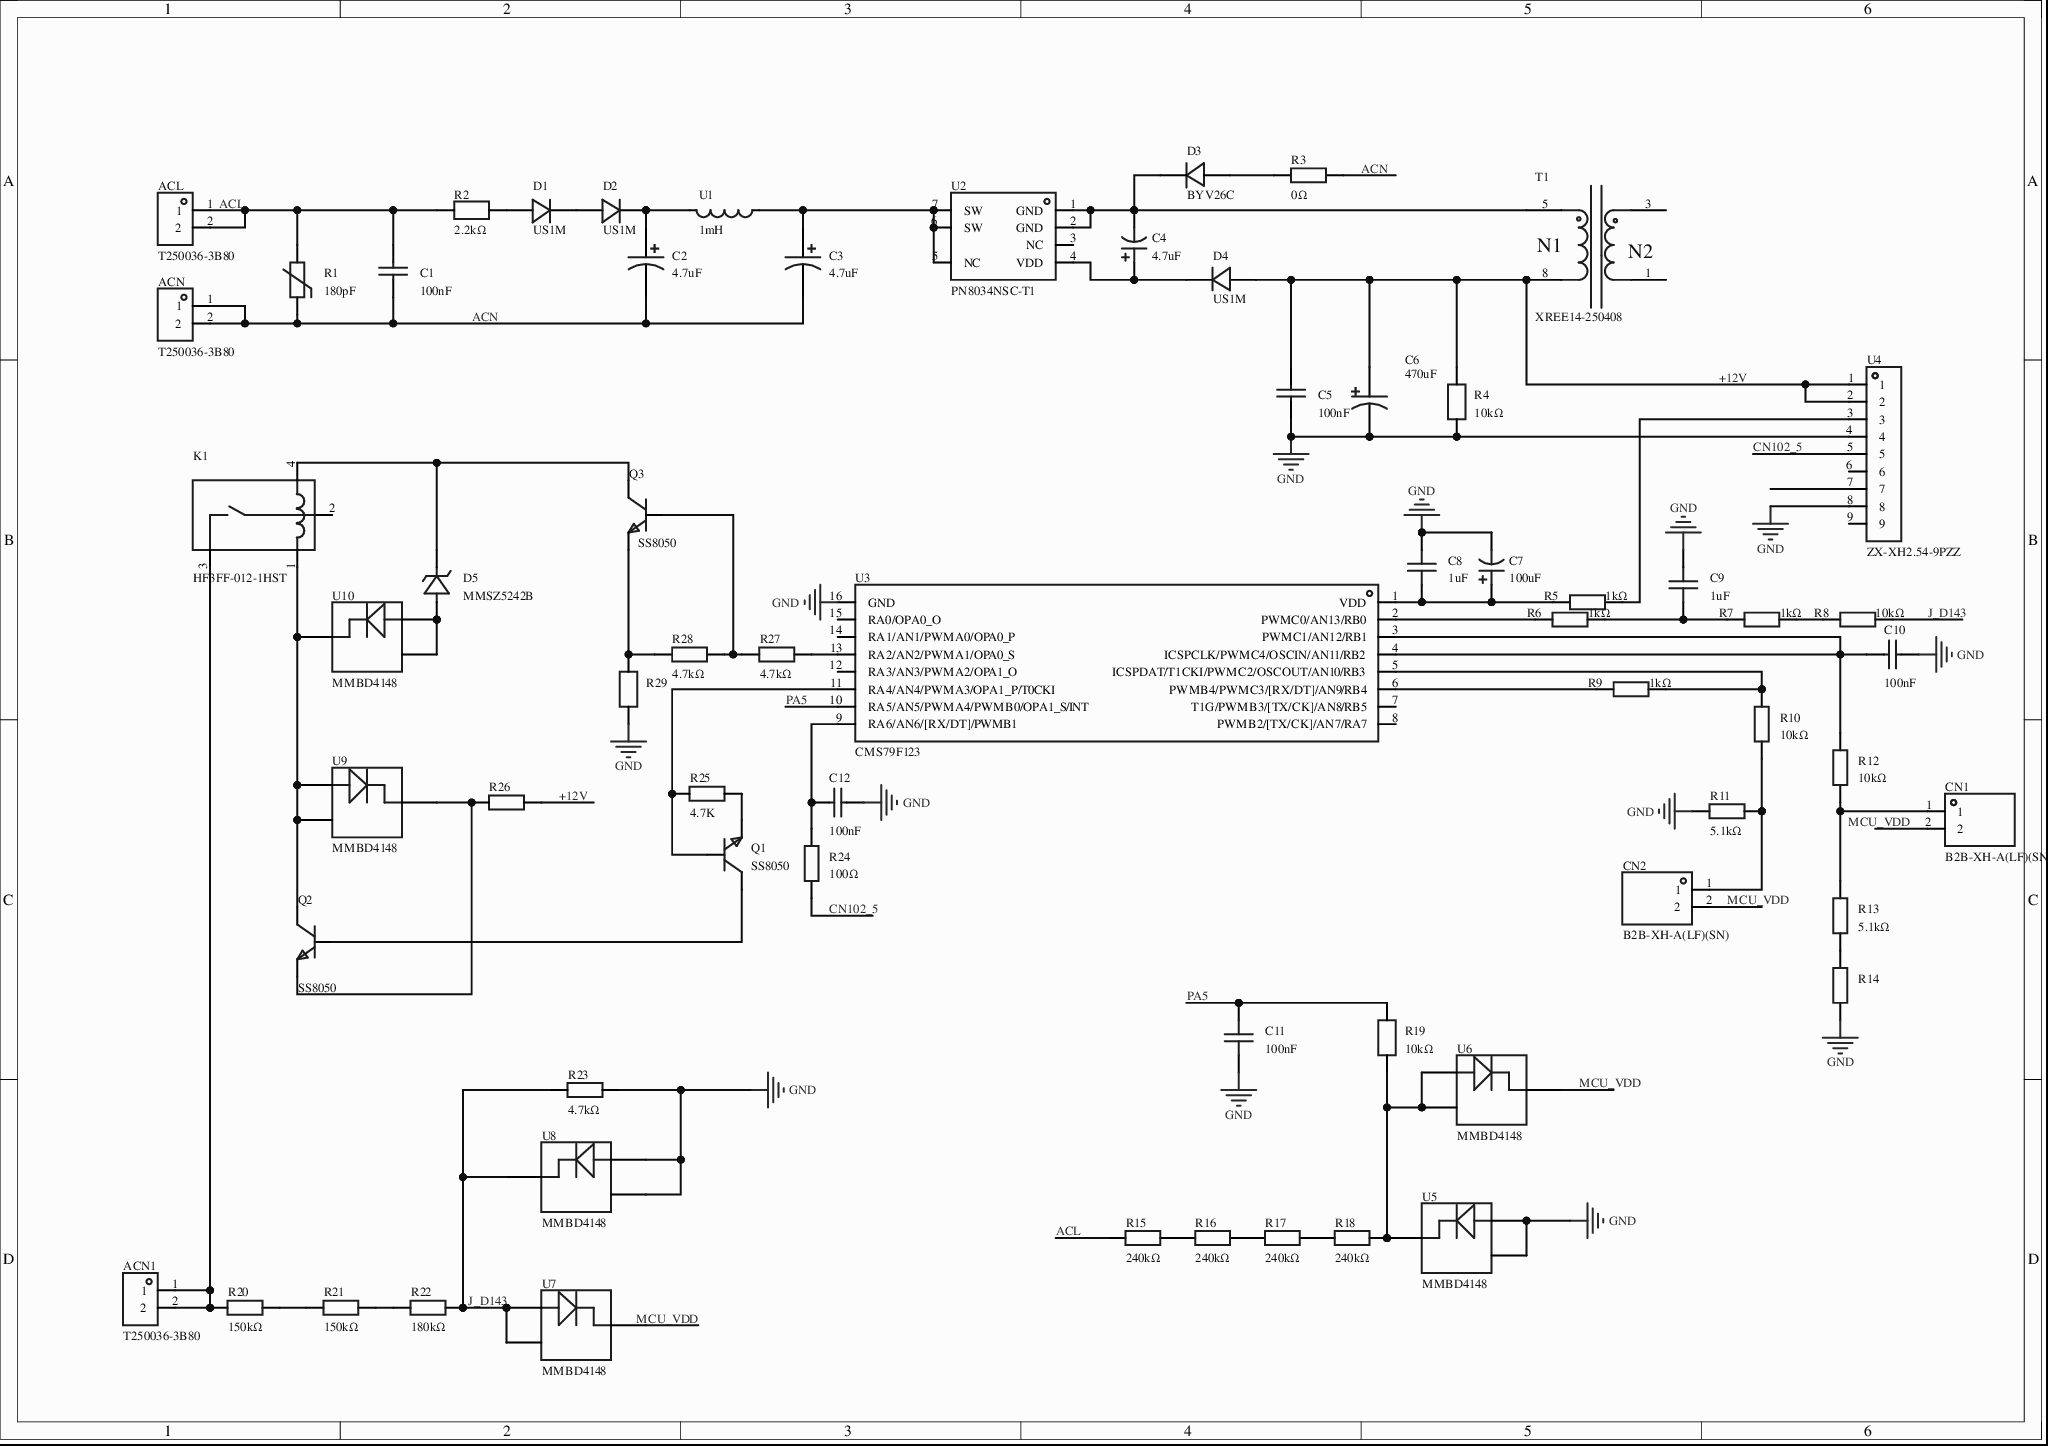
[diagram p0: MISC51809-3.schdoc]
# Altium project MISC51809-2.PrjPcb
1 sheet, 66 parts. Net scope: global (net labels, ports and power ports of the same name join across sheets).
Board file: MISC51809.pcbdoc

## Sheet MISC51809-3.schdoc
size 297 x 209 mm; Version: V1.0; @Project Name: MISC51809; @Update Date: 2026-04-03; @Create Date: 2026-04-03; @Board Name: MISC51809; @Create Time: 12:09:30; @Page Count: 1; @Page No: 1; @Schematic Name: MISC51809; @Update Time: 12:09:30; Size: A4

### Parts
ACL  T250036-3B80  [CONN-TH_XFCN-T250036-3B80]
ACN  T250036-3B80  [CONN-TH_XFCN-T250036-3B80]
ACN1  T250036-3B80  [CONN-TH_XFCN-T250036-3B80]
C1  100nF  [CAP-TH_L18.0-W6.0-P15.00-D1.2]
C2  4.7uF  [CAP-TH_BD10.0-P5.00-D1.0-FD]
C3  4.7uF  [CAP-TH_BD10.0-P5.00-D1.0-FD]
C4  4.7uF  [CAP-TH_BD6.3-P2.50-D0.5-FD]
C5  100nF  [C0603]
C6  470uF  [CAP-TH_BD10.0-P5.00-D1.0-FD]
C7  100uF  [CAP-TH_BD6.3-P2.50-D0.5-FD]
C8  1uF  [C0603]
C9  1uF  [C0603]
C10  100nF  [C0603]
C11  100nF  [C0603]
C12  100nF  [C0603]
CN1  B2B-XH-A(LF)(SN)  [CONN-TH_B2B-XH-A-LF-SN]
CN2  B2B-XH-A(LF)(SN)  [CONN-TH_B2B-XH-A-LF-SN]
D1  US1M  [SMA_L4.4-W2.8-LS5.4-RD]
D2  US1M  [SMA_L4.4-W2.8-LS5.4-RD]
D3  BYV26C  [SMA_L4.4-W2.6-LS5.1-FD]
D4  US1M  [SMA_L4.4-W2.8-LS5.4-RD]
D5  MMSZ5242B  [SOD-123_L2.7-W1.6-LS3.7-RD]
K1  HF3FF-012-1HST  [RELAY-TH_HF3FF-012-1HST]
Q1  SS8050  [SOT-23-3_L2.9-W1.3-P1.90-LS2.4-BR]
Q2  SS8050  [SOT-23-3_L2.9-W1.3-P1.90-LS2.4-BR]
Q3  SS8050  [SOT-23-3_L2.9-W1.3-P1.90-LS2.4-BR]
R1  180pF  [RES-TH_L11.0-W5.5-P7.50-D0.8-S4.70]
R2  2.2kΩ  [RES-TH_BD4.5-L11.5-P15.50-D0.8]
R3  0Ω  [R0805]
R4  10kΩ  [R0603]
R5  1kΩ  [R0603]
R6  1kΩ  [R0603]
R7  1kΩ  [R0603]
R8  10kΩ  [R0603]
R9  1kΩ  [R0603]
R10  10kΩ  [R0603]
R11  5.1kΩ  [R0603]
R12  10kΩ  [R0603]
R13  5.1kΩ  [R0603]
R14  1kΩ  [R0603]  (value not drawn)
R15  240kΩ  [R0805]
R16  240kΩ  [R0805]
R17  240kΩ  [R0805]
R18  240kΩ  [R0805]
R19  10kΩ  [R0603]
R20  150kΩ  [R0805]
R21  150kΩ  [R0805]
R22  180kΩ  [R0805]
R23  4.7kΩ  [RES-TH_BD3.3-L9.0-P13.00-D0.6]
R24  100Ω  [R0603]
R25  4.7K  [R0603]
R26  4.7K  [R0603]  (value not drawn)
R27  4.7kΩ  [R0603]
R28  4.7kΩ  [R0603]
R29  10kΩ  [R0603]  (value not drawn)
T1  XREE14-250408  [XFMR-TH_XREE14-250408]
U1  1mH  [IND-TH_BD3.0-L8.0-P12.00-D0.6]
U2  PN8034NSC-T1  [DIP-8_7P-L9.3-W6.4-P2.54-LS7.6-BL-PE6]
U3  CMS79F123  [SOPN-16_L9.9-W3.9-P1.27-LS6.0-BL]
U4  ZX-XH2.54-9PZZ  [CONN-TH_9P-P2.50_ZX-XH2.54-9PZZ]
U5  MMBD4148  [SOT-23-3_L2.9-W1.3-P1.90-LS2.4-BR]
U6  MMBD4148  [SOT-23-3_L2.9-W1.3-P1.90-LS2.4-BR]
U7  MMBD4148  [SOT-23-3_L2.9-W1.3-P1.90-LS2.4-BR]
U8  MMBD4148  [SOT-23-3_L2.9-W1.3-P1.90-LS2.4-BR]
U9  MMBD4148  [SOT-23-3_L2.9-W1.3-P1.90-LS2.4-BR]
U10  MMBD4148  [SOT-23-3_L2.9-W1.3-P1.90-LS2.4-BR]

### Nets
GND: C5.1 C6.2 C7.2 C8.2 C9.2 C10.1 C11.1 C12.2 R4.1 R11.2 R14.1 R23.2 R29.1 U3.16(GND) U4.4 U4.8 U5.1 U5.2 U8.1 U8.2
+12V: C5.2 C6.1 D4.2(A) R4.2 R26.2 T1.8 U4.1 U4.2
ACL: ACL.1 ACL.2 C1.2 R1.2 R2.1 R15.1
ACN: ACN.1 ACN.2 C1.1 C2.2 C3.2 R1.1 R3.2
CN102_5: R24.1 U4.5
J_D143: R8.2 R22.2 R23.1 U7.1 U7.2 U8.3
MCU_VDD: CN1.2 CN2.2 U6.3 U7.3
PA5: C11.2 R19.2 U3.10(RA5/AN5/PWMA4/PWMB0/OPA1_S/INT)
NetACN1_1: ACN1.1 ACN1.2 K1.3 R20.1
NetC2_1: C2.1 D2.1(C) U1.1
NetC3_1: C3.1 U1.2 U2.5(NC) U2.6(SW) U2.7(SW)
NetC4_1: C4.1 D4.1(C) U2.4(VDD)
NetC4_2: C4.2 D3.2 T1.5 U2.1(GND) U2.2(GND)
NetC7_1: C7.1 C8.1 R5.1 U3.1(VDD)
NetC9_1: C9.1 R6.2 R7.1
NetC10_2: C10.2 R12.2 U3.3(PWMC1/AN12/RB1) U3.4(ICSPCLK/PWMC4/OSCIN/AN11/RB2)
NetC12_1: C12.1 R24.2 U3.9(RA6/AN6/[RX/DT]/PWMB1)
NetCN1_1: CN1.1 R12.1 R13.1
NetCN2_1: CN2.1 R10.1 R11.1
NetD1_1: D1.1(C) D2.2(A)
NetD1_2: D1.2(A) R2.2
NetD3_1: D3.1 R3.1
NetD5_1: D5.1(K) K1.4 Q3.3(C)
NetD5_2: D5.2(A) U10.1 U10.2
NetK1_1: K1.1 Q2.3(C) U9.1 U9.2 U10.3
NetQ1_1: Q1.1(B) R25.1 U3.11(RA4/AN4/PWMA3/OPA1_P/T0CKI)
NetQ1_2: Q1.2(E) R25.2
NetQ1_3: Q1.3(C) Q2.1(B)
NetQ2_2: Q2.2(E) R26.1 U9.3
NetQ3_1: Q3.1(B) R27.1 R28.2
NetQ3_2: Q3.2(E) R28.1 R29.2
NetR5_2: R5.2 U4.3
NetR6_1: R6.1 U3.2(PWMC0/AN13/RB0)
NetR7_2: R7.2 R8.1
NetR9_1: R9.1 U3.6(PWMB4/PWMC3/[RX/DT]/AN9/RB4)
NetR9_2: R9.2 R10.2 U3.5(ICSPDAT/T1CKI/PWMC2/OSCOUT/AN10/RB3)
NetR13_2: R13.2 R14.2
NetR15_2: R15.2 R16.1
NetR16_2: R16.2 R17.1
NetR17_2: R17.2 R18.1
NetR18_2: R18.2 R19.1 U5.3 U6.1 U6.2
NetR20_2: R20.2 R21.1
NetR21_2: R21.2 R22.1
NetR27_2: R27.2 U3.13(RA2/AN2/PWMA1/OPA0_S)

Not connected (* = marked no-connect by the designer): K1 2; T1 1 3; U2 3(NC); U3 7(T1G/PWMB3/[TX/CK]/AN8/RB5) 8(PWMB2/[TX/CK]/AN7/RA7) 12(RA3/AN3/PWMA2/OPA1_O) 14(RA1/AN1/PWMA0/OPA0_P) 15(RA0/OPA0_O); U4 6 7 9

### Library data of the parts
ACL ACN ACN1 = T250036-3B80: 250 tab terminal, two pins; Manufacturer: XFCN(兴飞); AddInBom: yes; Symbol: T250036-3B80; Device: T250036-3B80; LCSC Part Name: T250036-3B80; SupplierPart: C42419908; ManufacturerPart: T250036-3B80; Supplier Footprint: 插件; JLCPCB Part Class: Extended Part; Datasheet: https://example.com/datasheet/T250036-3B80/44431582.html; Supplier: LCSC; ConvertToPcb: yes; FootprintName: CONN-TH_XFCN-T250036-3B80
C1 = MP2104K27D2X8LC: Capacitance:100nF;Tolerance:±10%;Working voltage(AC):275V;Safety class:X2;; Manufacturer: SRD(圣融达); Symbol: MP2104KGD2XLC; AddInBom: yes; ModelId: 72b0bd6426d647e6bc2e039f8f56a8da0819f05c4eef4c71ace90d822a990e87; ModelName: CAP-TH_L18.0-W6.0-H11.0-P15.0; ModelTransform: 708.66,236.22,0,0,0,0,0,0,-137.795; Tolerance: ±10%; Voltage(AC): 275V; Ratings: X2; safety certification: UL; ENEC; VDE; CQC; CSA; Device: MP2104K27D2X8LC; LCSC Part Name: 100nF ±10% 275V 等级:X2; SupplierPart: C105762; ManufacturerPart: MP2104K27D2X8LC; Supplier Footprint: 插件,P=15mm; JLCPCB Part Class: Extended Part; Datasheet: https://example.com/datasheet/MP2104K27D2X8LC/106977.html; Supplier: LCSC; ConvertToPcb: yes; FootprintName: CAP-TH_L18.0-W6.0-P15.00-D1.2; Value: 100nF
C2 C3 = 01EC1577SHG4.7uF450V: Capacitance:4.7uF;Tolerance:±20%;Rated voltage:450V;Ripple current:300mA@100kHz;Equivalent series resistance(ESR):3.5Ω@100kHz;; Manufacturer: KNSCHA(科尼盛); AddInBom: yes; ModelId: 6ce78ce5315348e095d700085da75e480819f05c4eef4c71ace90d822a990e87; ModelName: CAP-TH_D10.0-H16.0-P5.00; ModelTransform: 394.094,393.72252,0,0,0,0,0,0,-137.795; Tolerance: ±20%; Voltage Rating: 450V; Pin Spacing: 5mm; Lifetime: 5000hrs@105℃; Symbol: 01EC1577SHG4.7UF450V; Device: 01EC1577SHG4.7uF450V; LCSC Part Name: 4.7uF ±20% 450V; SupplierPart: C503212; ManufacturerPart: 01EC1577SHG4.7uF450V; Supplier Footprint: 插件,D10xL13mm; JLCPCB Part Class: Extended Part; Datasheet: https://example.com/datasheet/01EC1577SHG4.7uF450V/515625.html; Supplier: LCSC; ConvertToPcb: yes; FootprintName: CAP-TH_BD10.0-P5.00-D1.0-FD; Value: 4.7uF; Ripple Current: 300mA@100kHz; Equivalent Series Resistance(ESR): 3.5Ω@100kHz; Diameter: 10mm; Height - Seated (Max): 13mm; Operating Temperature: -40℃~+105℃
C4 = LKFC1101H4R7MF: Capacitance:4.7uF;Tolerance:±20%;Rated voltage:50V;; Manufacturer: Ymin(永铭); AddInBom: yes; ModelId: 983aa343eddc42b59ebb10541a88166e0819f05c4eef4c71ace90d822a990e87; ModelTransform: 247.99486,248.229,0,90,0,0,0,0,-196.85; Tolerance: ±20%; Voltage Rating: 50V; Symbol: LKFC1101H4R7MF; Device: LKFC1101H4R7MF; LCSC Part Name: 4.7uF ±20% 50V; SupplierPart: C19725777; ManufacturerPart: LKFC1101H4R7MF; Supplier Footprint: 插件,D6.3xL11mm; JLCPCB Part Class: Extended Part; Supplier: LCSC; ConvertToPcb: yes; FootprintName: CAP-TH_BD6.3-P2.50-D0.5-FD; ModelName: CAP-TH_BD6.3-P2.50-D0.5-FD; Value: 4.7uF; Diameter: 6.3mm; Height - Seated (Max): 11mm
C5 C10 C12 = CL10B104KA8NNNC: Capacitance:100nF;Tolerance:±10%;Rated voltage:25V;Temperature coefficient:X7R;; Manufacturer: SAMSUNG(三星); AddInBom: yes; ModelId: ac125912035d415993ca9572d50418b10819f05c4eef4c71ace90d822a990e87; ModelName: C0603_L1.6-W0.8-H0.8; ModelTransform: 62.992,31.496,0,0,0,0,0,0,0; Tolerance: ±10%; Voltage Rating: 25V; Temperature Coefficient: X7R; Symbol: CL10B104KA8NNNC; Device: CL10B104KA8NNNC; LCSC Part Name: 100nF ±10% 25V; SupplierPart: C1590; ManufacturerPart: CL10B104KA8NNNC; Supplier Footprint: 0603; JLCPCB Part Class: Extended Part; Datasheet: https://example.com/datasheet/CL10B104KA8NNNC/1942.html; Supplier: LCSC; ConvertToPcb: yes; FootprintName: C0603; Value: 100nF
C6 = RC025M471LO10*12TH-2A1E: Capacitance:470uF;Tolerance:±20%;Rated voltage:25V;Ripple current:950mA@100kHz;; Manufacturer: BERYL(绿宝石); AddInBom: yes; ModelId: 6ce78ce5315348e095d700085da75e480819f05c4eef4c71ace90d822a990e87; ModelName: CAP-TH_D10.0-H16.0-P5.00; ModelTransform: 394.094,393.72252,0,0,0,0,0,0,-137.795; Tolerance: ±20%; Voltage Rating: 25V; Pin Spacing: 5mm; Lifetime: 3000hrs@105℃; Symbol: RC025M471LO10*12TH-2A1E; Device: RC025M471LO10*12TH-2A1E; LCSC Part Name: 470uF ±20% 25V; SupplierPart: C365770; ManufacturerPart: RC025M471LO10*12TH-2A1E; Supplier Footprint: 插件,D10xL12mm; JLCPCB Part Class: Extended Part; Datasheet: https://example.com/upload/public/pdf/source/20190116/C365813_D032970E50E497412ED095DEE828BCD0.pdf; Supplier: LCSC; ConvertToPcb: yes; FootprintName: CAP-TH_BD10.0-P5.00-D1.0-FD; Value: 470uF; Ripple Current: 950mA@100kHz; Diameter: 10mm; Height - Seated (Max): 12mm; Operating Temperature: -40℃~+105℃
C7 = ERG25V100M6X7: Capacitance:100uF;Tolerance:±20%;Rated voltage:25V;; Manufacturer: JIERR(捷而瑞); AddInBom: yes; ModelId: 983aa343eddc42b59ebb10541a88166e0819f05c4eef4c71ace90d822a990e87; ModelTransform: 247.99486,248.229,0,90,0,0,0,0,-196.85; Tolerance: ±20%; Voltage Rating: 25V; Pin Spacing: 2.5mm; Lifetime: 2000hrs@105℃; Symbol: ERG25V100M6X7; Device: ERG25V100M6X7; LCSC Part Name: 100uF ±20% 25V; SupplierPart: C48935385; ManufacturerPart: ERG25V100M6X7; Supplier Footprint: 插件,D6.3xL7mm; JLCPCB Part Class: Extended Part; Datasheet: https://example.com/datasheet/ERG25V100M6X7/51248505.html; Supplier: LCSC; ConvertToPcb: yes; FootprintName: CAP-TH_BD6.3-P2.50-D0.5-FD; ModelName: CAP-TH_BD6.3-P2.50-D0.5-FD; Value: 100uF; Diameter: 6.3mm; Height - Seated (Max): 7mm; Operating Temperature: -40℃~+105℃
C8 C9 = CGA0603X5R105K250JT: Capacitance:1uF;Tolerance:±10%;Rated voltage:25V;Temperature coefficient:X5R;; Manufacturer: HRE(芯声); AddInBom: yes; ModelId: ac125912035d415993ca9572d50418b10819f05c4eef4c71ace90d822a990e87; ModelName: C0603_L1.6-W0.8-H0.8; ModelTransform: 62.992,31.496,0,0,0,0,0,0,0; Tolerance: ±10%; Voltage Rating: 25V; Temperature Coefficient: X5R; Symbol: CGA0603X5R105K250JT; Device: CGA0603X5R105K250JT; LCSC Part Name: 1uF ±10% 25V; SupplierPart: C6119818; ManufacturerPart: CGA0603X5R105K250JT; Supplier Footprint: 0603; JLCPCB Part Class: Extended Part; Datasheet: https://example.com/datasheet/CGA0603X5R105K250JT/7062524.html; Supplier: LCSC; ConvertToPcb: yes; FootprintName: C0603; Value: 1uF
C11 = CAP_0603: Symbol: Capacitance; ConvertToPcb: yes; ModelId: ac125912035d415993ca9572d50418b10819f05c4eef4c71ace90d822a990e87; ModelName: C0603_L1.6-W0.8-H0.8; ModelTransform: 62.992,31.496,0,0,0,0,0,0,0; Device: CAP_0603; AddInBom: yes; Supplier Footprint: 0603; FootprintName: C0603; Value: 100nF
CN1 CN2 = B2B-XH-A(LF)(SN): Pin structure:1x2P;Pitch:2.5mm;Mounting:Through-hole;Reference series:XH;Total pins:2P;Rows:1;Pins per row:2;Row spacing:-;Rated current:3A;Contact material:Brass;Contact plating:Tin;Operating temperature:-25℃~+85℃;; Manufacturer: JST; AddInBom: yes; ModelId: 2cd591bdb98c4759a6cba2f4f7745e410819f05c4eef4c71ace90d822a990e87; ModelName: XH2.5-2A; ModelTransform: 295.275,224.44837,0,180,0,0,0,18.701,-98.425; Pins Structure: 1x2P; Pitch: 2.5mm; Reference Series: XH; Number of PINs Per Row: 2; Current Rating: 3A; Voltage Rating: 250V; Plastic Material: PA66; Flame Retardant Rating: UL94V-0; Supplementary Features: Bent K pin; Z-Height of the Board: 7mm; X-Length of Bottom Edge on Board (Spacing Line): 7.4mm; Y-Width of Bottom Edge on Board: 5.75mm; Symbol: B2B-XH-A (LF)(SN); Device: B2B-XH-A(LF)(SN); LCSC Part Name: 1x2P 间距:2.5mm 直插 系列:XH; SupplierPart: C158012; ManufacturerPart: B2B-XH-A(LF)(SN); Supplier Footprint: 插件,P=2.5mm; JLCPCB Part Class: Extended Part; Datasheet: https://example.com/datasheet/B2B-XH-A(LF)(SN)/169360.html; Supplier: LCSC; ConvertToPcb: yes; FootprintName: CONN-TH_B2B-XH-A-LF-SN; Mounting Type: Through-hole; Number of Pins: 2P; Number of Rows: 1; Row Spacing: -; Contact Material: Brass; Contact Plating: Tin; Operating Temperature: -25℃~+85℃; Color: White
D1 D2 D4 = US1M_C412437: Diode configuration:Single;Forward voltage(Vf):1.65V@1A;DC reverse voltage(Vr):1kV;Rectified current:1A;Reverse recovery time(Trr):75ns;; Manufacturer: MDD(辰达半导体); Symbol: US1MG_C412437; AddInBom: yes; ModelId: 4f1e9ef2303f48b48aa8ce0cacf8d7b10819f05c4eef4c71ace90d822a990e87; ModelTransform: 204.724,102.362,0,0,0,0,0,0,0; Diode Configuration: Single; Voltage - DC Reverse(Vr): 1kV; Current - Rectified: 1A; Reverse Leakage Current (Ir): 5uA@1kV; Reverse Recovery Time (trr): 75ns; Operating Junction Temperature Range: -55℃~+150℃@(Tj); Non-Repetitive Peak Forward Surge Current: 30A; Device: US1M_C412437; LCSC Part Name: 耐压:1kV 电流:1A 反向恢复时间：75ns; SupplierPart: C412437; ManufacturerPart: US1M; Supplier Footprint: SMA; JLCPCB Part Class: Basic Part; Datasheet: https://example.com/datasheet/US1M/404260.html; Supplier: LCSC; ConvertToPcb: yes; FootprintName: SMA_L4.4-W2.8-LS5.4-RD; ModelName: SMA_L4.4-W2.8-LS5.4-RD; Voltage - Forward(Vf@If): 1.65V@1A
D3 = BYV26C_C2903924: Diode configuration:Single;Forward voltage(Vf):2.5V@1A;DC reverse voltage(Vr):600V;Rectified current:1A;Reverse recovery time(Trr):30ns;; Manufacturer: LGE(鲁光); AddInBom: yes; ModelId: 317f4ebd95d24908984f128fb0d4b37a0819f05c4eef4c71ace90d822a990e87; ModelTransform: 200.787,102.362,0,180,0,0,0,0,0; Diode Configuration: Single; Voltage - DC Reverse(Vr): 600V; Current - Rectified: 1A; Reverse Leakage Current (Ir): 5uA@600V; Reverse Recovery Time (trr): 30ns; Operating Junction Temperature Range: -55℃~+150℃@(Tj); Symbol: BYV26C_C2903924; Device: BYV26C_C2903924; LCSC Part Name: BYV26C; SupplierPart: C2903924; ManufacturerPart: BYV26C; Supplier Footprint: DO-214AC(SMA); JLCPCB Part Class: Extended Part; Datasheet: https://example.com/datasheet/BYV26C/3160962.html; Supplier: LCSC; ConvertToPcb: yes; FootprintName: SMA_L4.4-W2.6-LS5.1-FD; ModelName: SMA_L4.4-W2.6-LS5.1-FD; Voltage - Forward(Vf@If): 2.5V@1A
D5 = MMSZ5242B_C19077426: Diode configuration:Single;Zener voltage(nominal):12V;Zener voltage(range):11.4V~12.6V;Power dissipation(Pd):500mW;; Manufacturer: R+O(宏嘉诚); AddInBom: yes; ModelId: ad7e39f9e5534b3c96ffdc5532ebb4930819f05c4eef4c71ace90d822a990e87; ModelName: SOD-123_L2.7-W1.6-H1.4-LS3.7; ModelTransform: 146.026,62.992,0,180,0,0,0.0005,0,0; Diode Configuration: Single; Zener Voltage(Nom): 12V; Reverse Leakage Current (Ir): 1uA@9.1V; Pd - Power Dissipation: 500mW; Impedance(Zzt): 30Ω; Operating Junction Temperature Range: -55℃~+150℃; Symbol: MMSZ5242B_C19077426; Device: MMSZ5242B_C19077426; LCSC Part Name: 表面贴装齐纳二极管; SupplierPart: C19077426; ManufacturerPart: MMSZ5242B; Supplier Footprint: SOD-123; JLCPCB Part Class: Extended Part; Datasheet: https://example.com/datasheet/MMSZ5242B/20275511.html; Supplier: LCSC; ConvertToPcb: yes; FootprintName: SOD-123_L2.7-W1.6-LS3.7-RD; Zener Voltage(Range): 11.4V~12.6V
K1 = HF3FF-012-1HST: Coil voltage:12V;Contact form:One normally open group:1A(SPST-NO);Contact rating(resistive load):10A@28VDC;10A@277VAC;Max switching voltage:277V@AC;28V@DC;Max switching current:15A;; Manufacturer: HF(宏发); AddInBom: yes; ModelId: 2bf8f714452d4b7aae587b59869bcbd50819f05c4eef4c71ace90d822a990e87; ModelTransform: 748.03,598.424,0,0,0,0,39.369,0,-137.795; Coil Voltage: 12V; Coil Rated Power: 360mW; Switching Current(Max): 15A; Coil Type: Non-polar, single coil; Coil Resistance: 400Ω; Contact Resistance: 100mΩ; Operate Time: 10ms; Release Time: 5ms; Symbol: HF3FF-012-1HST; Device: HF3FF-012-1HST; LCSC Part Name: 超小型大功率12V继电器 单刀单掷-常开; SupplierPart: C329296; ManufacturerPart: HF3FF-012-1HST; Supplier Footprint: 插件,19x15.2mm; JLCPCB Part Class: Extended Part; Datasheet: https://example.com/datasheet/HF3FF-012-1HST/308957.html; Supplier: LCSC; ConvertToPcb: yes; FootprintName: RELAY-TH_HF3FF-012-1HST; ModelName: RELAY-TH_HF3FF-012-1HST; Contact Form: One normally open group:1A(SPST-NO); Number of Pins: 4; Contact Rating: 10A@28VDC; 10A@277VAC; Switching Voltage(Max): 277V@AC; 28V@DC; Contact Material: AgSnO2; Operating Temperature: -40℃~+85℃
Q1 Q2 = SS8050: Manufacturer: Doeshare(德芯); Symbol: SS8050_C2931717; AddInBom: yes; ModelId: c62791f0466c4ae2a892c056b845b0ca0819f05c4eef4c71ace90d822a990e87; ModelName: SOT-23-3P_L2.9-W1.3-H1.0-LS2.4-P0.95; ModelTransform: 98.425,114.173,0,180,0,0,0.0005,-0.0005,0; Device: SS8050; LCSC Part Name: NPN 25V 1.5A 120-400 SOT-23; SupplierPart: C2931717; ManufacturerPart: SS8050; Supplier Footprint: SOT-23; JLCPCB Part Class: Extended Part; Datasheet: https://example.com/upload/public/pdf/source/20220106/99F9A3DFCBDD91265C711555CE6390BF.pdf; Supplier: LCSC; ConvertToPcb: yes; FootprintName: SOT-23-3_L2.9-W1.3-P1.90-LS2.4-BR
Q3 = SS8050_C7420370: Transistor type:NPN;Collector current(Ic):1.5A;Collector-emitter breakdown voltage(Vceo):25V;Power dissipation(Pd):300mW;DC current gain(hFE):120@100mA,1.0V;; Manufacturer: R+O(宏嘉诚); AddInBom: yes; ModelId: c62791f0466c4ae2a892c056b845b0ca0819f05c4eef4c71ace90d822a990e87; ModelName: SOT-23-3P_L2.9-W1.3-H1.0-LS2.4-P0.95; ModelTransform: 98.425,114.173,0,180,0,0,0.0005,-0.0005,0; type: NPN; Current - Collector(Ic): 1.5A; Collector - Emitter Voltage VCEO: 25V; Pd - Power Dissipation: 300mW; Transition frequency(fT): 100MHz; Current - Collector Cutoff: 100nA; Vce Saturation(VCE(sat)): 500mV; Emitter-Base Voltage(Vebo): 5V; Symbol: SS8050_C7420370; Device: SS8050_C7420370; LCSC Part Name: H档 200-350 NPN 电流:1.5A 电压:25V; SupplierPart: C7420370; ManufacturerPart: SS8050; Supplier Footprint: SOT-23; JLCPCB Part Class: Extended Part; Datasheet: https://example.com/datasheet/SS8050/8397192.html; Supplier: LCSC; ConvertToPcb: yes; FootprintName: SOT-23-3_L2.9-W1.3-P1.90-LS2.4-BR; DC Current Gain: 120@100mA,1.0V; Operating Temperature: -55℃~+150℃
R1 = 10D561K_C49072850: Varistor voltage:504V~616V;Clamping voltage:920V;Working voltage(DC):460V;Working voltage(AC):350V;; Manufacturer: R+O(宏嘉诚); AddInBom: yes; ModelId: 2ac3a7b22a30408e97d27c4462d226650819f05c4eef4c71ace90d822a990e87; ModelName: RES-TH_L11.0-W5.5-H19.0-P7.50-D0.8-S5.50; ModelTransform: 433.0661,248.031,0,0,0,0,0,0,-196.85; Clamping Voltage: 920V; Maximum DC Volts: 460V; Maximum AC Volts: 350V; Peak Current: 2.5kA; Energy: 74J; Rated Wattage: 400mW; Symbol: 10D561K_C49072850; Device: 10D561K_C49072850; LCSC Part Name: 920V 74J; SupplierPart: C49072850; ManufacturerPart: 10D561K; Supplier Footprint: 插件,P=7.5mm; JLCPCB Part Class: Extended Part; Datasheet: https://example.com/datasheet/10D561K/51445316.html; Supplier: LCSC; ConvertToPcb: yes; FootprintName: RES-TH_L11.0-W5.5-P7.50-D0.8-S4.70; Varistor Voltage: 504V~616V; Value: 180pF
R2 = MF1W-2.2KΩ±1%T: Resistor type:Metal film resistor;Resistance:2.2kΩ;Tolerance:±1%;Power:1W;Temperature coefficient:±200ppm/℃;; Manufacturer: 华星机电; AddInBom: yes; ModelId: f1f7cfb3d56f4763951150e77c261d090819f05c4eef4c71ace90d822a990e87; ModelTransform: 641.73108,177.165,0,0,0,0,0,0,-196.85; Tolerance: ±1%; Power(Watts): 1W; Symbol: MF1W-2.2KΩ±1%T; Device: MF1W-2.2KΩ±1%T; LCSC Part Name: 金属膜电阻 2.2kΩ ±1% 1W; SupplierPart: C714107; ManufacturerPart: MF1W-2.2KΩ±1%T; Supplier Footprint: 插件,D4.5xL11.5mm; JLCPCB Part Class: Extended Part; Datasheet: https://example.com/upload/public/pdf/source/20200731/C713882_AE8EB1102749D7E4FB4FB13DC898C429.pdf; Supplier: LCSC; ConvertToPcb: yes; FootprintName: RES-TH_BD4.5-L11.5-P15.50-D0.8; ModelName: RES-TH_BD4.5-L11.5-P15.50-D0.8; Type: Metal film resistor; Value: 2.2kΩ; Temperature Coefficient: ±200ppm/℃
R3 = 0805W8F0000T5E: Resistor type:Thick film resistor;Resistance:0Ω;Tolerance:±1%;Power:125mW;Working voltage:150V;Temperature coefficient:±800ppm/℃;; Manufacturer: UNI-ROYAL(厚声); AddInBom: yes; ModelId: 37a81e68749a4138bd2dfa6897b24b850819f05c4eef4c71ace90d822a990e87; ModelName: R0805_L2.0-W1.3-H0.6; ModelTransform: 78.74,51.181,0,0,0,0,0,-0.0005,0; Tolerance: ±1%; Power(Watts): 125mW; Voltage-Supply(Max): 150V; Symbol: 0805W8F0000T5E; Device: 0805W8F0000T5E; LCSC Part Name: 0Ω ±1% 125mW 厚膜电阻; SupplierPart: C17477; ManufacturerPart: 0805W8F0000T5E; Supplier Footprint: 0805; JLCPCB Part Class: Basic Part; Datasheet: https://example.com/datasheet/0805W8F0000T5E/18165.html; Supplier: LCSC; ConvertToPcb: yes; FootprintName: R0805; Type: Thick film resistor; Value: 0Ω; Temperature Coefficient: ±800ppm/℃; Operating Temperature: -55℃~+155℃
R4 R19 R29 = FRC0603F1002TS: Resistor type:Thick film resistor;Resistance:10kΩ;Tolerance:±1%;Power:100mW;Working voltage:75V;Temperature coefficient:±100ppm/℃;; Manufacturer: FOJAN(富捷); AddInBom: yes; ModelId: fc143cca1e79419f9cd78b61e9279f080819f05c4eef4c71ace90d822a990e87; ModelTransform: 31.8897,63.7794,0,90,0,0,0,0,0; Tolerance: ±1%; Power(Watts): 100mW; Voltage-Supply(Max): 75V; Symbol: FRC0603F1002TS; Device: FRC0603F1002TS; LCSC Part Name: 10kΩ ±1% 100mW 厚膜电阻; SupplierPart: C2906982; ManufacturerPart: FRC0603F1002TS; Supplier Footprint: 0603; JLCPCB Part Class: Extended Part; Supplier: LCSC; ConvertToPcb: yes; FootprintName: R0603; ModelName: R0603; Type: Thick film resistor; Value: 10kΩ; Temperature Coefficient: ±100ppm/℃; Operating Temperature: -55℃~+155℃
R5-R14 = 0603WAF1001T5E: Resistor type:Thick film resistor;Resistance:1kΩ;Tolerance:±1%;Power:100mW;Working voltage:75V;Temperature coefficient:±100ppm/℃;; Manufacturer: UNI-ROYAL(厚声); AddInBom: yes; ModelId: fc143cca1e79419f9cd78b61e9279f080819f05c4eef4c71ace90d822a990e87; ModelTransform: 31.8897,63.7794,0,90,0,0,0,0,0; Tolerance: ±1%; Power(Watts): 100mW; Voltage-Supply(Max): 75V; Symbol: 0603WAF1001T5E; Device: 0603WAF1001T5E; LCSC Part Name: 1kΩ ±1% 100mW 厚膜电阻; ManufacturerPart: 0603WAF1001T5E; Supplier Footprint: 0603; JLCPCB Part Class: Basic Part; Datasheet: https://example.com/datasheet/0603WAF1001T5E/21904.html; Supplier: LCSC; ConvertToPcb: yes; FootprintName: R0603; ModelName: R0603; Type: Thick film resistor; Temperature Coefficient: ±100ppm/℃; Operating Temperature: -55℃~+155℃
  R5-R7 R9 R14: SupplierPart: C21190; Value: 1kΩ
  R8 R10 R12: Value: 10kΩ
  R11 R13: Value: 5.1kΩ
R15-R18 = 0805W8F2403T5E: Resistor type:Thick film resistor;Resistance:240kΩ;Tolerance:±1%;Power:125mW;Working voltage:150V;Temperature coefficient:±100ppm/℃;; Manufacturer: UNI-ROYAL(厚声); AddInBom: yes; ModelId: 37a81e68749a4138bd2dfa6897b24b850819f05c4eef4c71ace90d822a990e87; ModelName: R0805_L2.0-W1.3-H0.6; ModelTransform: 78.74,51.181,0,0,0,0,0,-0.0005,0; Tolerance: ±1%; Power(Watts): 125mW; Voltage-Supply(Max): 150V; Symbol: 0805W8F2403T5E; Device: 0805W8F2403T5E; LCSC Part Name: 240kΩ ±1% 125mW 厚膜电阻; SupplierPart: C25824; ManufacturerPart: 0805W8F2403T5E; Supplier Footprint: 0805; JLCPCB Part Class: Extended Part; Datasheet: https://example.com/datasheet/0805W8F2403T5E/26567.html; Supplier: LCSC; ConvertToPcb: yes; FootprintName: R0805; Type: Thick film resistor; Value: 240kΩ; Temperature Coefficient: ±100ppm/℃; Operating Temperature: -55℃~+155℃
R20 R21 = 0805W8F1503T5E: Resistor type:Thick film resistor;Resistance:150kΩ;Tolerance:±1%;Power:125mW;Max working voltage:150V;Temperature coefficient:±100ppm/℃;; Manufacturer: UNI-ROYAL(厚声); AddInBom: yes; ModelId: 37a81e68749a4138bd2dfa6897b24b850819f05c4eef4c71ace90d822a990e87; ModelName: R0805_L2.0-W1.3-H0.6; ModelTransform: 78.74,51.181,0,0,0,0,0,-0.0005,0; Tolerance: ±1%; Power(Watts): 125mW; Overload Voltage (Max): 150V; Symbol: 0805W8F1503T5E; Device: 0805W8F1503T5E; LCSC Part Name: 150kΩ ±1% 125mW 厚膜电阻; SupplierPart: C17470; ManufacturerPart: 0805W8F1503T5E; Supplier Footprint: 0805; JLCPCB Part Class: Basic Part; Datasheet: https://example.com/upload/public/pdf/source/20200306/C422600_1E6D84923E4A46A82E41ADD87F860B5C.pdf; Supplier: LCSC; ConvertToPcb: yes; FootprintName: R0805; Type: Thick film resistor; Value: 150kΩ; Temperature Coefficient: ±100ppm/℃; Operating Temperature Range: -55℃~+155℃
R22 = 0805W8F1803T5E: Resistor type:Thick film resistor;Resistance:180kΩ;Tolerance:±1%;Power:125mW;Max working voltage:150V;Temperature coefficient:±100ppm/℃;; Manufacturer: UNI-ROYAL(厚声); AddInBom: yes; ModelId: 37a81e68749a4138bd2dfa6897b24b850819f05c4eef4c71ace90d822a990e87; ModelName: R0805_L2.0-W1.3-H0.6; ModelTransform: 78.74,51.181,0,0,0,0,0,-0.0005,0; Tolerance: ±1%; Power(Watts): 125mW; Overload Voltage (Max): 150V; Symbol: 0805W8F1803T5E; Device: 0805W8F1803T5E; LCSC Part Name: 180kΩ ±1% 125mW 厚膜电阻; SupplierPart: C17501; ManufacturerPart: 0805W8F1803T5E; Supplier Footprint: 0805; JLCPCB Part Class: Extended Part; Datasheet: https://example.com/upload/public/pdf/source/20200306/C422600_1E6D84923E4A46A82E41ADD87F860B5C.pdf; Supplier: LCSC; ConvertToPcb: yes; FootprintName: R0805; Type: Thick film resistor; Value: 180kΩ; Temperature Coefficient: ±100ppm/℃; Operating Temperature Range: -55℃~+155℃
R23 = RN1WS4.7KΩFT/BA1: Resistor type:Metal film resistor;Resistance:4.7kΩ;Tolerance:±1%;Power:1W;Temperature coefficient:±50ppm/℃;; Manufacturer: Tyohm(幸亚电阻); AddInBom: yes; ModelId: ba6d6a4d684e4c9c99cd35ba00f099d90819f05c4eef4c71ace90d822a990e87; ModelTransform: 535.432,129.82565,0,0,0,0,0,0,-196.85; Tolerance: ±1%; Power(Watts): 1W; Symbol: RN1WS4.7KΩFT/BA1; Device: RN1WS4.7KΩFT/BA1; LCSC Part Name: 4.7kΩ ±1% 1W 金属膜电阻; SupplierPart: C385387; ManufacturerPart: RN1WS4.7KΩFT/BA1; Supplier Footprint: 插件,D3.3xL9.2mm; JLCPCB Part Class: Extended Part; Datasheet: https://example.com/datasheet/RN1WS4.7K%25CE%25A9FT/BA1/359234.html; Supplier: LCSC; ConvertToPcb: yes; FootprintName: RES-TH_BD3.3-L9.0-P13.00-D0.6; ModelName: RES-TH_BD3.3-L9.0-P13.00-D0.6; Type: Metal film resistor; Value: 4.7kΩ; Temperature Coefficient: ±50ppm/℃
R24 = RC0603FR-07100RL: Resistor type:Thick film resistor;Resistance:100Ω;Tolerance:±1%;Power:100mW;Max working voltage:75V;Temperature coefficient:±100ppm/℃;; Manufacturer: YAGEO(国巨); AddInBom: yes; ModelId: fc143cca1e79419f9cd78b61e9279f080819f05c4eef4c71ace90d822a990e87; ModelTransform: 31.8897,63.7794,0,90,0,0,0,0,0; Tolerance: ±1%; Power(Watts): 100mW; Overload Voltage (Max): 75V; Symbol: RC0603FR-07100RL; Device: RC0603FR-07100RL; LCSC Part Name: 厚膜电阻 100Ω ±1% 100mW; SupplierPart: C105588; ManufacturerPart: RC0603FR-07100RL; Supplier Footprint: 0603; JLCPCB Part Class: Extended Part; Datasheet: https://example.com/upload/public/pdf/source/20180316/70C0E2BDAE7FCC62C531A5A58D202EE1.pdf; Supplier: LCSC; ConvertToPcb: yes; FootprintName: R0603; ModelName: R0603; Type: Thick film resistor; Value: 100Ω; Temperature Coefficient: ±100ppm/℃; Operating Temperature Range: -55℃~+155℃
R25 R26 = Res_0603: Symbol: Resistor; ConvertToPcb: yes; ModelId: fc143cca1e79419f9cd78b61e9279f080819f05c4eef4c71ace90d822a990e87; ModelTransform: 31.8897,63.7794,0,90,0,0,0,0,0; Device: Res_0603; Value: 4.7K; AddInBom: yes; Supplier Footprint: 0603; FootprintName: R0603; ModelName: R0603
R27 R28 = 0603WAF4701T5E: Resistor type:Thick film resistor;Resistance:4.7kΩ;Tolerance:±1%;Power:100mW;Working voltage:75V;Temperature coefficient:±100ppm/℃;; Manufacturer: UNI-ROYAL(厚声); AddInBom: yes; ModelId: fc143cca1e79419f9cd78b61e9279f080819f05c4eef4c71ace90d822a990e87; ModelTransform: 31.8897,63.7794,0,90,0,0,0,0,0; Tolerance: ±1%; Power(Watts): 100mW; Voltage-Supply(Max): 75V; Symbol: 0603WAF4701T5E; Device: 0603WAF4701T5E; LCSC Part Name: 4.7kΩ ±1% 100mW 厚膜电阻; SupplierPart: C23162; ManufacturerPart: 0603WAF4701T5E; Supplier Footprint: 0603; JLCPCB Part Class: Basic Part; Datasheet: https://example.com/datasheet/0603WAF4701T5E/23889.html; Supplier: LCSC; ConvertToPcb: yes; FootprintName: R0603; ModelName: R0603; Type: Thick film resistor; Value: 4.7kΩ; Temperature Coefficient: ±100ppm/℃; Operating Temperature: -55℃~+155℃
T1 = XREE14-250408: Inductance:1.0mH@@Test condition:10KHZ 0.3V@@Withstand voltage test:P--C1000V/5mA/60S; Manufacturer: XR(祥如); AddInBom: yes; Symbol: XREE14-250408; Device: XREE14-250408; LCSC Part Name: XREE14  立式  4+4  1.0mH; SupplierPart: C48391659; ManufacturerPart: XREE14-250408; Supplier Footprint: 插件; JLCPCB Part Class: Extended Part; Datasheet: https://example.com/datasheet/XREE14-250408/50640744.html; Supplier: LCSC; ConvertToPcb: yes; FootprintName: XFMR-TH_XREE14-250408
U1 = YAL0307-102K: Inductance:1mH;Tolerance:±10%;Rated current:60mA;Saturation current(Isat):-;Type:Color-ring inductor;Q factor:60@0.796MHz;; Manufacturer: YJYCOIN(益嘉源); AddInBom: yes; ModelId: 2b1f7f9f49994586afa140ea54b99bdf0819f05c4eef4c71ace90d822a990e87; ModelTransform: 496.062,118.11,0,0,0,0,0,0,-216.535; Tolerance: ±10%; Current Rating: 60mA; DC Resistance(DCR): 30Ω; Frequency - Self Resonant: 1.2MHz; Symbol: YAL0307-102K; Device: YAL0307-102K; LCSC Part Name: 1mH ±10% 色环电感; SupplierPart: C514869; ManufacturerPart: YAL0307-102K; Supplier Footprint: 插件,D3xL8mm; JLCPCB Part Class: Extended Part; Datasheet: https://example.com/datasheet/YAL0307-102K/530158.html; Supplier: LCSC; ConvertToPcb: yes; FootprintName: IND-TH_BD3.0-L8.0-P12.00-D0.6; ModelName: IND-TH_BD3.0-L8.0-P12.00-D0.6; Value: 1mH; Current - Saturation(Isat): -; Type: Color-ring inductor; Q @ Frequency: 60@0.796MHz; Ratings: -
U2 = PN8034NSC-T1: Working voltage:10V~20V;Switching frequency:-;Output current:300mA;Transistor voltage rating:650V;; Manufacturer: chipown(芯朋微电子); AddInBom: yes; ModelId: 82d0c570693840b98e7f854f091680580819f05c4eef4c71ace90d822a990e87; ModelTransform: 364.173,309.842,0,0,0,0,0,0,-118.11; Isolation: Non-isolated; Output Current: 300mA; Voltage - Breakdown: 650V; Topology: Buck-boost;Buck; Working Mode: CCM; DCM; Output Voltage: 12V; Symbol: PN8034NSC-T1; Device: PN8034NSC-T1; LCSC Part Name: 650V 10V~20V 300mA; SupplierPart: C163040; ManufacturerPart: PN8034NSC-T1; Supplier Footprint: DIP-7; JLCPCB Part Class: Extended Part; Datasheet: https://example.com/datasheet/PN8034NSC-T1/174421.html; Supplier: LCSC; ConvertToPcb: yes; FootprintName: DIP-8_7P-L9.3-W6.4-P2.54-LS7.6-BL-PE6; ModelName: DIP-8_7P-L9.3-W6.4-P2.54-LS7.6-BL-PE6; Voltage - Supply: 10V~20V; Frequency - Switching: -; Pd - Power Dissipation: -; Duty Cycle(Max): -; Features: Over-temperature protection(OTP);Under-voltage protection(UVP);Over-current protection(OCP); Operating Temperature: -40℃~+150℃; Feedback System: -
U3 = CMS79F123: AddInBom: yes; ModelId: 4386bda0e236455db33deb57599145450819f05c4eef4c71ace90d822a990e87; ModelName: SOPN-16_L9.9-W3.9-H1.8-LS6.0-P1.27; ModelTransform: 389.763,236.22,0,0,0,0,0,0,0; Symbol: CMS79F123; Device: CMS79F123; LCSC Part Name: CMS79F123; SupplierPart: C9900011040; ManufacturerPart: CMS79F123; Supplier Footprint: SOPN-16-150mil; JLCPCB Part Class: Extended Part; Supplier: LCSC; ConvertToPcb: yes; FootprintName: SOPN-16_L9.9-W3.9-P1.27-LS6.0-BL
U4 = ZX-XH2.54-9PZZ: Pin structure:1x9P;Pitch:2.5mm;Mounting:Through-hole;Reference series:XH;Total pins:9P;Rows:1;Pins per row:9;Row spacing:-;Rated current:2A;Contact material:Brass;Contact plating:Tin;Operating temperature:-25℃~+85℃;; Manufacturer: Megastar(兆星); AddInBom: yes; ModelId: 68c85730bd154dda8e395768ec9a93b60819f05c4eef4c71ace90d822a990e87; ModelTransform: 984.25,232.6767,0,0,0,0,0,21.378,-133.858; Pins Structure: 1x9P; Pitch: 2.5mm; Reference Series: XH; Number of PINs Per Row: 9; Current Rating: 2A; Voltage Rating: 250V; Plastic Material: PA66; Flame Retardant Rating: UL94V-0; Z-Height of the Board: 7mm; X-Length of Bottom Edge on Board (Spacing Line): 25mm; Y-Width of Bottom Edge on Board: 5.9mm; Symbol: ZX-XH2.54-9PZZ; Device: ZX-XH2.54-9PZZ; LCSC Part Name: 1x9P 间距:2.5mm 直插 系列:XH; SupplierPart: C7429639; ManufacturerPart: ZX-XH2.54-9PZZ; Supplier Footprint: 插件,P=2.5mm; JLCPCB Part Class: Extended Part; Datasheet: https://example.com/datasheet/ZX-XH2.54-9PZZ/8427556.html; Supplier: LCSC; ConvertToPcb: yes; FootprintName: CONN-TH_9P-P2.50_ZX-XH2.54-9PZZ; ModelName: CONN-TH_9P-P2.50_ZX-XH2.54-9PZZ; Mounting Type: Through-hole; Number of Pins: 9P; Number of Rows: 1; Row Spacing: -; Contact Material: Brass; Contact Plating: Tin; Operating Temperature: -25℃~+85℃; Supplementary Features: -; Color: White
U5-U10 = MMBD4148_C7461109: Forward voltage(Vf):1.25V@150mA;DC reverse voltage(Vr):75V;Rectified current:150mA;Reverse recovery time(Trr):4ns;; Manufacturer: BORN(伯恩半导体); AddInBom: yes; ModelId: c62791f0466c4ae2a892c056b845b0ca0819f05c4eef4c71ace90d822a990e87; ModelName: SOT-23-3P_L2.9-W1.3-H1.0-LS2.4-P0.95; ModelTransform: 98.425,114.173,0,180,0,0,0.0005,-0.0005,0; Voltage - DC Reverse(Vr): 75V; Current - Rectified: 150mA; Pd - Power Dissipation: 350mW; Reverse Leakage Current (Ir): 2.5uA@75V; Reverse Recovery Time (trr): 4ns; Operating Junction Temperature Range: -55℃~+150℃; Non-Repetitive Peak Forward Surge Current: 2A; Symbol: MMBD4148_C7461109; Device: MMBD4148_C7461109; LCSC Part Name: 75V 150mA; SupplierPart: C7461109; ManufacturerPart: MMBD4148; Supplier Footprint: SOT-23; JLCPCB Part Class: Extended Part; Datasheet: https://example.com/datasheet/MMBD4148/8488516.html; Supplier: LCSC; ConvertToPcb: yes; FootprintName: SOT-23-3_L2.9-W1.3-P1.90-LS2.4-BR; Voltage - Forward(Vf@If): 1.25V@150mA